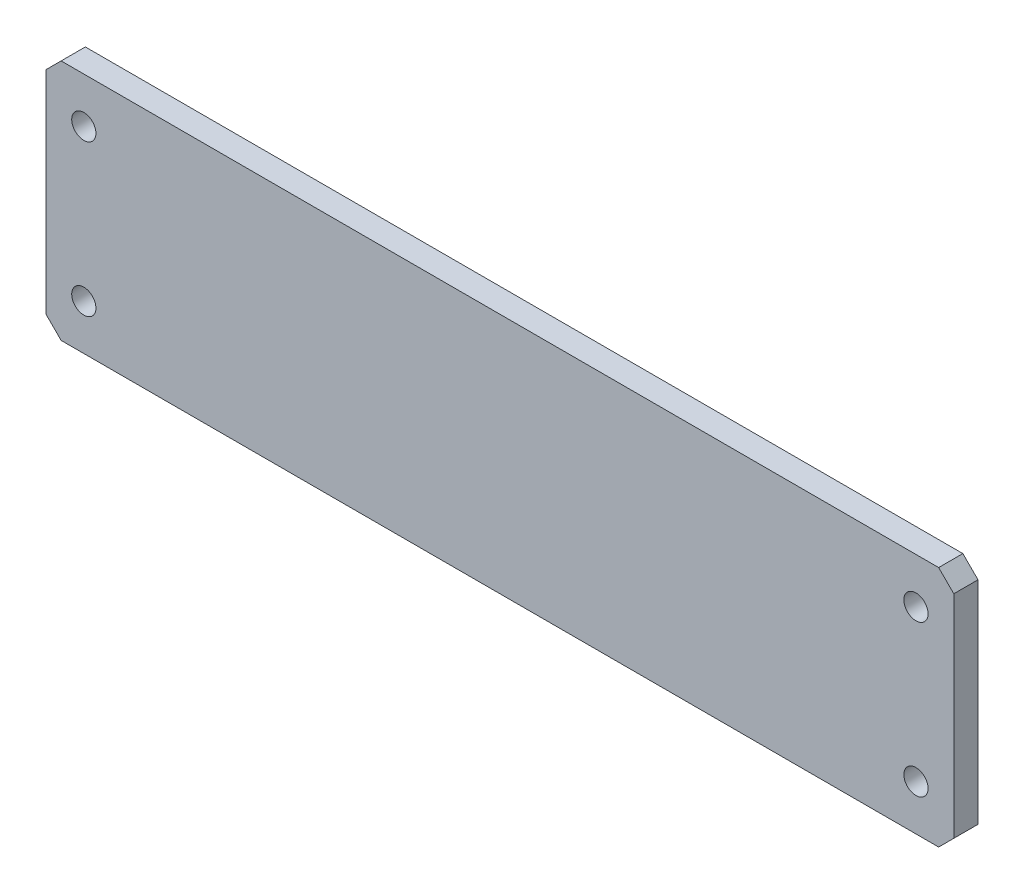
SolidWorks part; units mm, degrees
material "1023 carbon steel plate (SS)"
ref_plane "Front Plane" through (0, 0, 0) normal (0, 0, 1) x (1, 0, 0)
ref_plane "Top Plane" through (0, 0, 0) normal (0, 1, 0) x (1, 0, 0)
ref_plane "Right Plane" through (0, 0, 0) normal (1, 0, 0) x (0, 0, -1)
sketch "Sketch1" plane through (0, 0, 0) normal (0, 0, 1) x (1, 0, 0)
  line L1 (-150, 40) -> (150, 40)
  line L2 (-150, 40) -> (-150, -40)
  line L3 (-150, -40) -> (150, -40)
  line L4 (150, 40) -> (150, -40)
  line L5 (-150, 40) -> (150, -40) construction
  line L6 (-150, -40) -> (150, 40) construction
  point P0 (0, 0)
  dimension "D1" = 300
  dimension "D2" = 80
extrude "Boss-Extrude1" add sketch "Sketch1" along normal blind 8 contours L2 L1 L4 L3
sketch "Sketch2" plane through (0, 0, 8) normal (0, 0, 1) x (1, 0, 0)
  line L0 (-150, 40) -> (-150, -40) construction
  line L1 (-150, 40) -> (150, 40) construction
  circle A0 centre (-137.5, 25) radius 4
  circle A1 centre (-137.5, -25) radius 4
  circle A2 centre (137.5, 25) radius 4
  circle A3 centre (137.5, -25) radius 4
  dimension "D5" = 8
  dimension "D1" = 275
  dimension "D2" = 50
  dimension "D3" = 12.5
  dimension "D4" = 15
extrude "Cut-Extrude1" cut sketch "Sketch2" against normal blind 8
chamfer "Chamfer1" distance 5 angle 45 4 edges at (150, 40, 4) (150, -40, 4) (-150, -40, 4) (-150, 40, 4)
